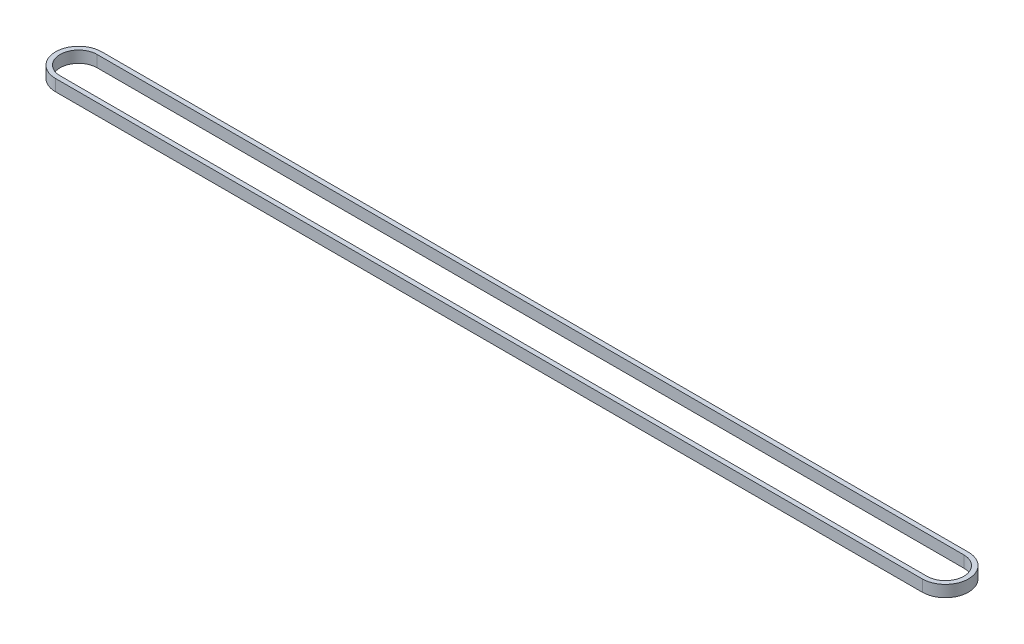
SolidWorks part; units mm, degrees
ref_plane "Front Plane" through (0, 0, 0) normal (0, 0, 1) x (1, 0, 0)
ref_plane "Top Plane" through (0, 0, 0) normal (0, 1, 0) x (1, 0, 0)
ref_plane "Right Plane" through (0, 0, 0) normal (1, 0, 0) x (0, 0, -1)
sketch "Sketch1" plane through (0, 0, 0) normal (0, 1, 0) x (1, 0, 0)
  line L0 (-348.9594, 0) -> (26.0406, 0) construction
  line L1 (-348.9594, 8) -> (26.0406, 8)
  line L2 (-348.9594, -8) -> (26.0406, -8)
  line L3 (-348.9594, 10) -> (26.0406, 10)
  line L4 (-348.9594, -10) -> (26.0406, -10)
  arc A0 (-348.9594, 8) -> (-348.9594, -8) centre (-348.9594, 0) ccw
  arc A1 (26.0406, -8) -> (26.0406, 8) centre (26.0406, 0) ccw
  arc A2 (26.0406, -10) -> (26.0406, 10) centre (26.0406, 0) ccw
  arc A3 (-348.9594, 10) -> (-348.9594, -10) centre (-348.9594, 0) ccw
  point P3 (-161.4594, 0)
  dimension "D1" = 8
  dimension "D3" = 375
  dimension "D2" = 2
extrude "Boss-Extrude1" add sketch "Sketch1" along normal blind 5
